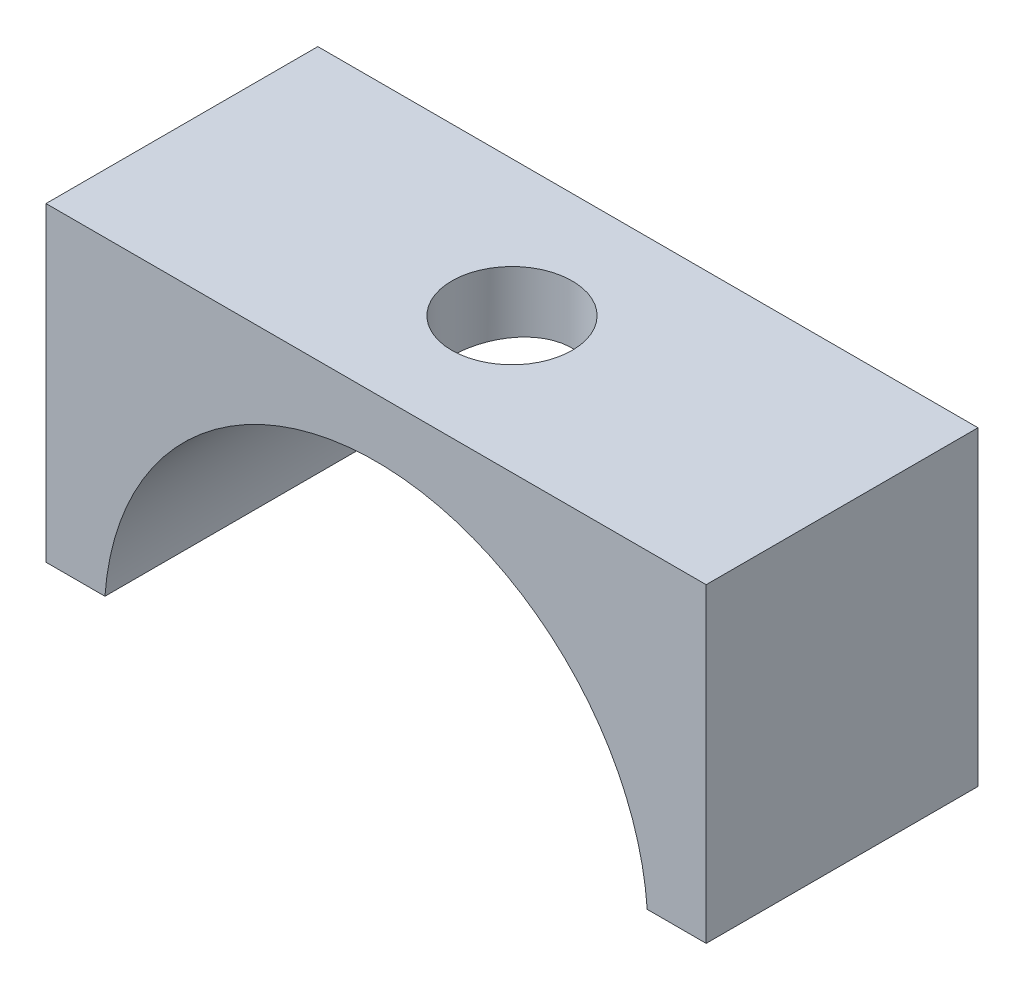
SolidWorks part; units mm, degrees
material "尼龙 101"
ref_plane "前视基准面" through (0, 0, 0) normal (0, 0, 1) x (1, 0, 0)
ref_plane "上视基准面" through (0, 0, 0) normal (0, 1, 0) x (1, 0, 0)
ref_plane "右视基准面" through (0, 0, 0) normal (1, 0, 0) x (0, 0, -1)
other "Configuration Table"
sketch "草图1" plane through (0, 0, 0) normal (0, 0, 1) x (1, 0, 0)
  line L0 (0, 0) -> (21.2753, 0) construction
  line L1 (-8.5, 8.5) -> (8.5, 8.5)
  line L2 (-8.5, 8.5) -> (-8.5, -8.5)
  line L3 (-8.5, -8.5) -> (8.5, -8.5)
  line L4 (8.5, 8.5) -> (8.5, -8.5)
  line L5 (-8.5, 8.5) -> (8.5, -8.5) construction
  line L6 (-8.5, -8.5) -> (8.5, 8.5) construction
  line L7 (0, 0) -> (0, 22.157) construction
  line L8 (-12.2746, 0.5) -> (17.5956, 0.5)
  circle A0 centre (0, 0) radius 7
  point P0 (0, 0)
  dimension "D2" = 14
  dimension "D1" = 17
  dimension "D3" = 0.5
extrude "凸台-拉伸1" add sketch "草图1" along normal blind 7 contours A0 L8 L4 L1 L2
sketch "草图2" plane through (0, 8.5, 0) normal (0, 1, 0) x (1, 0, 0)
  line L0 (-8.5, 0) -> (8.5, 0) construction
  circle A0 centre (0, -3.5) radius 1.55
  dimension "D1" = 3.1
  dimension "D2" = 3.5
extrude "切除-拉伸1" cut sketch "草图2" against normal blind 7
